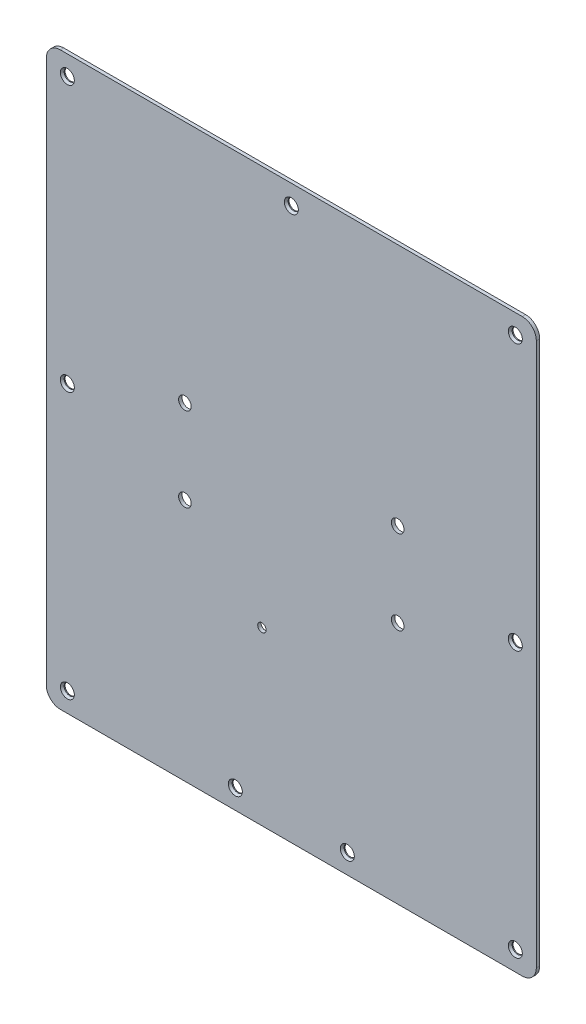
SolidWorks part; units mm, degrees
ref_plane "Front Plane" through (0, 0, 0) normal (0, 0, 1) x (1, 0, 0)
ref_plane "Top Plane" through (0, 0, 0) normal (0, 1, 0) x (1, 0, 0)
ref_plane "Right Plane" through (0, 0, 0) normal (1, 0, 0) x (0, 0, -1)
sketch "Model" plane through (0, 0, 0) normal (0, 0, 1) x (1, 0, 0)
  line L65 (0, -102) -> (82.5, -102)
  line L66 (0, 99.3974) -> (0, 90.6765) construction
  line L67 (-4.7436, 95) -> (4.0628, 95) construction
  line L68 (0, 102) -> (82.5, 102)
  line L69 (80, 4.4344) -> (80, -4.2865) construction
  line L70 (75.2564, 95) -> (84.0628, 95) construction
  line L71 (80, 99.3974) -> (80, 90.6765) construction
  line L72 (80, 4.3974) -> (80, -4.3235) construction
  line L73 (75.2564, 0) -> (84.0628, 0) construction
  line L74 (80, -99.3974) -> (80, -90.6765) construction
  line L75 (75.2564, -95) -> (84.0628, -95) construction
  line L76 (15.2564, -95) -> (24.0628, -95) construction
  line L77 (20, -99.3974) -> (20, -90.6765) construction
  line L78 (-20, -99.3974) -> (-20, -90.6765) construction
  line L79 (-15.2564, -95) -> (-24.0628, -95) construction
  line L80 (-75.2564, -95) -> (-84.0628, -95) construction
  line L81 (-80, -99.3974) -> (-80, -90.6765) construction
  line L82 (-75.2564, 0) -> (-84.0628, 0) construction
  line L83 (-80, 4.3974) -> (-80, -4.3235) construction
  line L84 (-80, 99.3974) -> (-80, 90.6765) construction
  line L86 (-80, 4.4344) -> (-80, -4.2865) construction
  line L87 (0, 102) -> (-82.5, 102)
  line L88 (0, -102) -> (-82.5, -102)
  line L89 (34.2836, 15) -> (41.7164, 15) construction
  line L90 (38, 18.7164) -> (38, 11.2836) construction
  line L91 (-38, 18.7164) -> (-38, 11.2836) construction
  line L92 (-34.2836, 15) -> (-41.7164, 15) construction
  line L137 (-38, -18.7164) -> (-38, -11.2836) construction
  line L138 (-34.2836, -15) -> (-41.7164, -15) construction
  line L139 (38, -18.7164) -> (38, -11.2836) construction
  line L140 (34.2836, -15) -> (41.7164, -15) construction
  line L141 (-87.5, 97) -> (-87.5, -97)
  line L142 (87.5, 97) -> (87.5, -97)
  line L153 (-10.5, -40.7) -> (-6, -40.7) construction
  line L154 (-10.5, -40.7) -> (-10.5, -36.2) construction
  line L155 (-10.5, -40.7) -> (-15, -40.7) construction
  line L156 (-10.5, -40.7) -> (-10.5, -45.2) construction
  circle A2 centre (0, 95) radius 2
  circle A3 centre (0, 95.037) radius 3.8
  circle A4 centre (80, 95.037) radius 3.8
  circle A5 centre (80, 95) radius 2
  circle A6 centre (80, 0) radius 2
  circle A7 centre (80, 0.037) radius 3.8
  circle A8 centre (80, -95) radius 2
  circle A9 centre (80, -95.037) radius 3.8
  circle A10 centre (20, -95.037) radius 3.8
  circle A11 centre (20, -95) radius 2
  circle A12 centre (-20, -95) radius 2
  circle A13 centre (-20, -95.037) radius 3.8
  circle A14 centre (-80, -95.037) radius 3.8
  circle A15 centre (-80, -95) radius 2
  circle A16 centre (-80, 0.037) radius 3.8
  circle A17 centre (-80, 0) radius 2
  circle A18 centre (-80, 95) radius 2
  circle A20 centre (38, 15) radius 2.25
  circle A21 centre (-38, 15) radius 2.25
  circle A22 centre (-38, -15) radius 2.25
  circle A23 centre (38, -15) radius 2.25
  arc A24 (-87.5, -97) -> (-82.5, -102) centre (-82.5, -97) ccw
  arc A25 (-82.5, 102) -> (-87.5, 97) centre (-82.5, 97) ccw
  arc A26 (82.5, -102) -> (87.5, -97) centre (82.5, -97) ccw
  arc A27 (87.5, 97) -> (82.5, 102) centre (82.5, 97) ccw
  circle A29 centre (-10.5, -40.7) radius 1.5
extrude "Boss-Extrude1" add sketch "Model" along normal blind 1.2 contours A18 | A2 | A5 | A6 | A21 | A22 | A17 | A15 | A12 | A11 | A8 | A23
chamfer "Chamfer1" distance 0.5 angle 60 9 edges at (-78, -95, 1.2) (-18, -95, 1.2) (22, -95, 1.2) (82, -95, 1.2) (82, 0, 1.2) (-78, 0, 1.2) (82, 95, 1.2) (2, 95, 1.2) (-78, 95, 1.2)
sketch "Sketch2" plane through (0, 0, 0) normal (0, 0, -1) x (-1, 0, 0)
  circle A0 centre (0, 0) radius 1.9
  dimension "D1" = 3.8
extrude "Boss-Extrude2" add sketch "Sketch2" along normal blind 30
chamfer "Chamfer2" distance 0.5 angle 60 1 edges at (-1.9, 0, -30)
sketch "Sketch3" plane through (0, 0, -30) normal (0, 0, -1) x (-1, 0, 0)
  circle A0 centre (0, 0) radius 1.9
curve "Helix/Spiral1" pitch 1 height 29.25 turns 29.25
sketch "Sketch4" plane through (0, 0, 0) normal (0, 1, 0) x (1, 0, 0)
  line L0 (-1.9, 30) -> (-1.9, 21.2581) construction
  line L1 (-1.9, 29.5) -> (-1.9, 0) construction
  line L2 (-1.9, 30) -> (2.0958, 30) construction
  line L3 (-1.91, 30.4) -> (-1.91, 29.6)
  line L4 (-1.91, 29.6) -> (-1.5636, 29.8)
  line L5 (-1.5636, 29.8) -> (-1.5636, 30.2)
  line L6 (-1.5636, 30.2) -> (-1.91, 30.4)
  spline S0 degree 3 poles (-1.9, 30) (-1.9, 29.9793) (-1.8011, 29.9374) (-1.3785, 29.875) (-0.746, 29.8125) (0, 29.75) (0.746, 29.6875) (1.3785, 29.625) (1.8011, 29.5625) (1.9495, 29.5) (1.8011, 29.4375) (1.3785, 29.375) (0.746, 29.3125) (0, 29.25) (-0.746, 29.1875) (-1.3785, 29.125) (-1.8011, 29.0625) (-1.9495, 29) (-1.8011, 28.9375) (-1.3785, 28.875) (-0.746, 28.8125) (0, 28.75) (0.746, 28.6875) (1.3785, 28.625) (1.8011, 28.5625) (1.9495, 28.5) (1.8011, 28.4375) (1.3785, 28.375) (0.746, 28.3125) (0, 28.25) (-0.746, 28.1875) (-1.3785, 28.125) (-1.8011, 28.0625) (-1.9495, 28) (-1.8011, 27.9375) (-1.3785, 27.875) (-0.746, 27.8125) (0, 27.75) (0.746, 27.6875) (1.3785, 27.625) (1.8011, 27.5625) (1.9495, 27.5) (1.8011, 27.4375) (1.3785, 27.375) (0.746, 27.3125) (0, 27.25) (-0.746, 27.1875) (-1.3785, 27.125) (-1.8011, 27.0625) (-1.9495, 27) (-1.8011, 26.9375) (-1.3785, 26.875) (-0.746, 26.8125) (0, 26.75) (0.746, 26.6875) (1.3785, 26.625) (1.8011, 26.5625) (1.9495, 26.5) (1.8011, 26.4375) (1.3785, 26.375) (0.746, 26.3125) (0, 26.25) (-0.746, 26.1875) (-1.3785, 26.125) (-1.8011, 26.0625) (-1.9495, 26) (-1.8011, 25.9375) (-1.3785, 25.875) (-0.746, 25.8125) (0, 25.75) (0.746, 25.6875) (1.3785, 25.625) (1.8011, 25.5625) (1.9495, 25.5) (1.8011, 25.4375) (1.3785, 25.375) (0.746, 25.3125) (0, 25.25) (-0.746, 25.1875) (-1.3785, 25.125) (-1.8011, 25.0625) (-1.9495, 25) (-1.8011, 24.9375) (-1.3785, 24.875) (-0.746, 24.8125) (0, 24.75) (0.746, 24.6875) (1.3785, 24.625) (1.8011, 24.5625) (1.9495, 24.5) (1.8011, 24.4375) (1.3785, 24.375) (0.746, 24.3125) (0, 24.25) (-0.746, 24.1875) (-1.3785, 24.125) (-1.8011, 24.0625) (-1.9495, 24) (-1.8011, 23.9375) (-1.3785, 23.875) (-0.746, 23.8125) (0, 23.75) (0.746, 23.6875) (1.3785, 23.625) (1.8011, 23.5625) (1.9495, 23.5) (1.8011, 23.4375) (1.3785, 23.375) (0.746, 23.3125) (0, 23.25) (-0.746, 23.1875) (-1.3785, 23.125) (-1.8011, 23.0625) (-1.9495, 23) (-1.8011, 22.9375) (-1.3785, 22.875) (-0.746, 22.8125) (0, 22.75) (0.746, 22.6875) (1.3785, 22.625) (1.8011, 22.5625) (1.9495, 22.5) (1.8011, 22.4375) (1.3785, 22.375) (0.746, 22.3125) (0, 22.25) (-0.746, 22.1875) (-1.3785, 22.125) (-1.8011, 22.0625) (-1.9495, 22) (-1.8011, 21.9375) (-1.3785, 21.875) (-0.746, 21.8125) (0, 21.75) (0.746, 21.6875) (1.3785, 21.625) (1.8011, 21.5625) (1.9495, 21.5) (1.8011, 21.4375) (1.3785, 21.375) (0.746, 21.3125) (0, 21.25) (-0.746, 21.1875) (-1.3785, 21.125) (-1.8011, 21.0625) (-1.9495, 21) (-1.8011, 20.9375) (-1.3785, 20.875) (-0.746, 20.8125) (0, 20.75) (0.746, 20.6875) (1.3785, 20.625) (1.8011, 20.5625) (1.9495, 20.5) (1.8011, 20.4375) (1.3785, 20.375) (0.746, 20.3125) (0, 20.25) (-0.746, 20.1875) (-1.3785, 20.125) (-1.8011, 20.0625) (-1.9495, 20) (-1.8011, 19.9375) (-1.3785, 19.875) (-0.746, 19.8125) (0, 19.75) (0.746, 19.6875) (1.3785, 19.625) (1.8011, 19.5625) (1.9495, 19.5) (1.8011, 19.4375) (1.3785, 19.375) (0.746, 19.3125) (0, 19.25) (-0.746, 19.1875) (-1.3785, 19.125) (-1.8011, 19.0625) (-1.9495, 19) (-1.8011, 18.9375) (-1.3785, 18.875) (-0.746, 18.8125) (0, 18.75) (0.746, 18.6875) (1.3785, 18.625) (1.8011, 18.5625) (1.9495, 18.5) (1.8011, 18.4375) (1.3785, 18.375) (0.746, 18.3125) (0, 18.25) (-0.746, 18.1875) (-1.3785, 18.125) (-1.8011, 18.0625) (-1.9495, 18) (-1.8011, 17.9375) (-1.3785, 17.875) (-0.746, 17.8125) (0, 17.75) (0.746, 17.6875) (1.3785, 17.625) (1.8011, 17.5625) (1.9495, 17.5) (1.8011, 17.4375) (1.3785, 17.375) (0.746, 17.3125) (0, 17.25) (-0.746, 17.1875) (-1.3785, 17.125) (-1.8011, 17.0625) (-1.9495, 17) (-1.8011, 16.9375) (-1.3785, 16.875) (-0.746, 16.8125) (0, 16.75) (0.746, 16.6875) (1.3785, 16.625) (1.8011, 16.5625) (1.9495, 16.5) (1.8011, 16.4375) (1.3785, 16.375) (0.746, 16.3125) (0, 16.25) (-0.746, 16.1875) (-1.3785, 16.125) (-1.8011, 16.0625) (-1.9495, 16) (-1.8011, 15.9375) (-1.3785, 15.875) (-0.746, 15.8125) (0, 15.75) (0.746, 15.6875) (1.3785, 15.625) (1.8011, 15.5625) (1.9495, 15.5) (1.8011, 15.4375) (1.3785, 15.375) (0.746, 15.3125) (0, 15.25) (-0.746, 15.1875) (-1.3785, 15.125) (-1.8011, 15.0625) (-1.9495, 15) (-1.8011, 14.9375) (-1.3785, 14.875) (-0.746, 14.8125) (0, 14.75) (0.746, 14.6875) (1.3785, 14.625) (1.8011, 14.5625) (1.9495, 14.5) (1.8011, 14.4375) (1.3785, 14.375) (0.746, 14.3125) (0, 14.25) (-0.746, 14.1875) (-1.3785, 14.125) (-1.8011, 14.0625) (-1.9495, 14) (-1.8011, 13.9375) (-1.3785, 13.875) (-0.746, 13.8125) (0, 13.75) (0.746, 13.6875) (1.3785, 13.625) (1.8011, 13.5625) (1.9495, 13.5) (1.8011, 13.4375) (1.3785, 13.375) (0.746, 13.3125) (0, 13.25) (-0.746, 13.1875) (-1.3785, 13.125) (-1.8011, 13.0625) (-1.9495, 13) (-1.8011, 12.9375) (-1.3785, 12.875) (-0.746, 12.8125) (0, 12.75) (0.746, 12.6875) (1.3785, 12.625) (1.8011, 12.5625) (1.9495, 12.5) (1.8011, 12.4375) (1.3785, 12.375) (0.746, 12.3125) (0, 12.25) (-0.746, 12.1875) (-1.3785, 12.125) (-1.8011, 12.0625) (-1.9495, 12) (-1.8011, 11.9375) (-1.3785, 11.875) (-0.746, 11.8125) (0, 11.75) (0.746, 11.6875) (1.3785, 11.625) (1.8011, 11.5625) (1.9495, 11.5) (1.8011, 11.4375) (1.3785, 11.375) (0.746, 11.3125) (0, 11.25) (-0.746, 11.1875) (-1.3785, 11.125) (-1.8011, 11.0625) (-1.9495, 11) (-1.8011, 10.9375) (-1.3785, 10.875) (-0.746, 10.8125) (0, 10.75) (0.746, 10.6875) (1.3785, 10.625) (1.8011, 10.5625) (1.9495, 10.5) (1.8011, 10.4375) (1.3785, 10.375) (0.746, 10.3125) (0, 10.25) (-0.746, 10.1875) (-1.3785, 10.125) (-1.8011, 10.0625) (-1.9495, 10) (-1.8011, 9.9375) (-1.3785, 9.875) (-0.746, 9.8125) (0, 9.75) (0.746, 9.6875) (1.3785, 9.625) (1.8011, 9.5625) (1.9495, 9.5) (1.8011, 9.4375) (1.3785, 9.375) (0.746, 9.3125) (0, 9.25) (-0.746, 9.1875) (-1.3785, 9.125) (-1.8011, 9.0625) (-1.9495, 9) (-1.8011, 8.9375) (-1.3785, 8.875) (-0.746, 8.8125) (0, 8.75) (0.746, 8.6875) (1.3785, 8.625) (1.8011, 8.5625) (1.9495, 8.5) (1.8011, 8.4375) (1.3785, 8.375) (0.746, 8.3125) (0, 8.25) (-0.746, 8.1875) (-1.3785, 8.125) (-1.8011, 8.0625) (-1.9495, 8) (-1.8011, 7.9375) (-1.3785, 7.875) (-0.746, 7.8125) (0, 7.75) (0.746, 7.6875) (1.3785, 7.625) (1.8011, 7.5625) (1.9495, 7.5) (1.8011, 7.4375) (1.3785, 7.375) (0.746, 7.3125) (0, 7.25) (-0.746, 7.1875) (-1.3785, 7.125) (-1.8011, 7.0625) (-1.9495, 7) (-1.8011, 6.9375) (-1.3785, 6.875) (-0.746, 6.8125) (0, 6.75) (0.746, 6.6875) (1.3785, 6.625) (1.8011, 6.5625) (1.9495, 6.5) (1.8011, 6.4375) (1.3785, 6.375) (0.746, 6.3125) (0, 6.25) (-0.746, 6.1875) (-1.3785, 6.125) (-1.8011, 6.0625) (-1.9495, 6) (-1.8011, 5.9375) (-1.3785, 5.875) (-0.746, 5.8125) (0, 5.75) (0.746, 5.6875) (1.3785, 5.625) (1.8011, 5.5625) (1.9495, 5.5) (1.8011, 5.4375) (1.3785, 5.375) (0.746, 5.3125) (0, 5.25) (-0.746, 5.1875) (-1.3785, 5.125) (-1.8011, 5.0625) (-1.9495, 5) (-1.8011, 4.9375) (-1.3785, 4.875) (-0.746, 4.8125) (0, 4.75) (0.746, 4.6875) (1.3785, 4.625) (1.8011, 4.5625) (1.9495, 4.5) (1.8011, 4.4375) (1.3785, 4.375) (0.746, 4.3125) (0, 4.25) (-0.746, 4.1875) (-1.3785, 4.125) (-1.8011, 4.0625) (-1.9495, 4) (-1.8011, 3.9375) (-1.3785, 3.875) (-0.746, 3.8125) (0, 3.75) (0.746, 3.6875) (1.3785, 3.625) (1.8011, 3.5625) (1.9495, 3.5) (1.8011, 3.4375) (1.3785, 3.375) (0.746, 3.3125) (0, 3.25) (-0.746, 3.1875) (-1.3785, 3.125) (-1.8011, 3.0625) (-1.9495, 3) (-1.8011, 2.9375) (-1.3785, 2.875) (-0.746, 2.8125) (0, 2.75) (0.746, 2.6875) (1.3785, 2.625) (1.8011, 2.5625) (1.9495, 2.5) (1.8011, 2.4375) (1.3785, 2.375) (0.746, 2.3125) (0, 2.25) (-0.746, 2.1875) (-1.3785, 2.125) (-1.8011, 2.0625) (-1.9495, 2) (-1.8011, 1.9375) (-1.3785, 1.875) (-0.746, 1.8125) (0, 1.75) (0.746, 1.6875) (1.3785, 1.625) (1.8011, 1.5625) (1.9495, 1.5) (1.8011, 1.4375) (1.3785, 1.375) (0.746, 1.3125) (0, 1.25) (-0.746, 1.1875) (-1.3785, 1.125) (-1.8011, 1.0625) (-1.9495, 1) (-1.8011, 0.9375) (-1.3783, 0.875) (-0.7467, 0.8126) (-0.2471, 0.7707) (0, 0.75) knots 0 0 0 0 0.002137 0.004274 0.00641 0.008547 0.010684 0.012821 0.014957 0.017094 0.019231 0.021368 0.023504 0.025641 0.027778 0.029915 0.032051 0.034188 0.036325 0.038462 0.040598 0.042735 0.044872 0.047009 0.049145 0.051282 0.053419 0.055556 0.057692 0.059829 0.061966 0.064103 0.066239 0.068376 0.070513 0.07265 0.074786 0.076923 0.07906 0.081197 0.083333 0.08547 0.087607 0.089744 0.09188 0.094017 0.096154 0.098291 0.100427 0.102564 0.104701 0.106838 0.108974 0.111111 0.113248 0.115385 0.117521 0.119658 0.121795 0.123932 0.126068 0.128205 0.130342 0.132479 0.134615 0.136752 0.138889 0.141026 0.143162 0.145299 0.147436 0.149573 0.151709 0.153846 0.155983 0.15812 0.160256 0.162393 0.16453 0.166667 0.168803 0.17094 0.173077 0.175214 0.17735 0.179487 0.181624 0.183761 0.185897 0.188034 0.190171 0.192308 0.194444 0.196581 0.198718 0.200855 0.202991 0.205128 0.207265 0.209402 0.211538 0.213675 0.215812 0.217949 0.220085 0.222222 0.224359 0.226496 0.228632 0.230769 0.232906 0.235043 0.237179 0.239316 0.241453 0.24359 0.245726 0.247863 0.25 0.252137 0.254274 0.25641 0.258547 0.260684 0.262821 0.264957 0.267094 0.269231 0.271368 0.273504 0.275641 0.277778 0.279915 0.282051 0.284188 0.286325 0.288462 0.290598 0.292735 0.294872 0.297009 0.299145 0.301282 0.303419 0.305556 0.307692 0.309829 0.311966 0.314103 0.316239 0.318376 0.320513 0.32265 0.324786 0.326923 0.32906 0.331197 0.333333 0.33547 0.337607 0.339744 0.34188 0.344017 0.346154 0.348291 0.350427 0.352564 0.354701 0.356838 0.358974 0.361111 0.363248 0.365385 0.367521 0.369658 0.371795 0.373932 0.376068 0.378205 0.380342 0.382479 0.384615 0.386752 0.388889 0.391026 0.393162 0.395299 0.397436 0.399573 0.401709 0.403846 0.405983 0.40812 0.410256 0.412393 0.41453 0.416667 0.418803 0.42094 0.423077 0.425214 0.42735 0.429487 0.431624 0.433761 0.435897 0.438034 0.440171 0.442308 0.444444 0.446581 0.448718 0.450855 0.452991 0.455128 0.457265 0.459402 0.461538 0.463675 0.465812 0.467949 0.470085 0.472222 0.474359 0.476496 0.478632 0.480769 0.482906 0.485043 0.487179 0.489316 0.491453 0.49359 0.495726 0.497863 0.5 0.502137 0.504274 0.50641 0.508547 0.510684 0.512821 0.514957 0.517094 0.519231 0.521368 0.523504 0.525641 0.527778 0.529915 0.532051 0.534188 0.536325 0.538462 0.540598 0.542735 0.544872 0.547009 0.549145 0.551282 0.553419 0.555556 0.557692 0.559829 0.561966 0.564103 0.566239 0.568376 0.570513 0.57265 0.574786 0.576923 0.57906 0.581197 0.583333 0.58547 0.587607 0.589744 0.59188 0.594017 0.596154 0.598291 0.600427 0.602564 0.604701 0.606838 0.608974 0.611111 0.613248 0.615385 0.617521 0.619658 0.621795 0.623932 0.626068 0.628205 0.630342 0.632479 0.634615 0.636752 0.638889 0.641026 0.643162 0.645299 0.647436 0.649573 0.651709 0.653846 0.655983 0.65812 0.660256 0.662393 0.66453 0.666667 0.668803 0.67094 0.673077 0.675214 0.67735 0.679487 0.681624 0.683761 0.685897 0.688034 0.690171 0.692308 0.694444 0.696581 0.698718 0.700855 0.702991 0.705128 0.707265 0.709402 0.711538 0.713675 0.715812 0.717949 0.720085 0.722222 0.724359 0.726496 0.728632 0.730769 0.732906 0.735043 0.737179 0.739316 0.741453 0.74359 0.745726 0.747863 0.75 0.752137 0.754274 0.75641 0.758547 0.760684 0.762821 0.764957 0.767094 0.769231 0.771368 0.773504 0.775641 0.777778 0.779915 0.782051 0.784188 0.786325 0.788462 0.790598 0.792735 0.794872 0.797009 0.799145 0.801282 0.803419 0.805556 0.807692 0.809829 0.811966 0.814103 0.816239 0.818376 0.820513 0.82265 0.824786 0.826923 0.82906 0.831197 0.833333 0.83547 0.837607 0.839744 0.84188 0.844017 0.846154 0.848291 0.850427 0.852564 0.854701 0.856838 0.858974 0.861111 0.863248 0.865385 0.867521 0.869658 0.871795 0.873932 0.876068 0.878205 0.880342 0.882479 0.884615 0.886752 0.888889 0.891026 0.893162 0.895299 0.897436 0.899573 0.901709 0.903846 0.905983 0.90812 0.910256 0.912393 0.91453 0.916667 0.918803 0.92094 0.923077 0.925214 0.92735 0.929487 0.931624 0.933761 0.935897 0.938034 0.940171 0.942308 0.944444 0.946581 0.948718 0.950855 0.952991 0.955128 0.957265 0.959402 0.961538 0.963675 0.965812 0.967949 0.970085 0.972222 0.974359 0.976496 0.978632 0.980769 0.982906 0.985043 0.987179 0.989316 0.991453 0.99359 0.995726 0.997863 1 1 1 1 construction
  dimension "D1" = 0.8
  dimension "D2" = 0.01
  dimension "D3" = 0.4
  dimension "D4" = 60
sweep "Cut-Sweep1" cut profiles "Sketch4" path "Helix/Spiral1"
